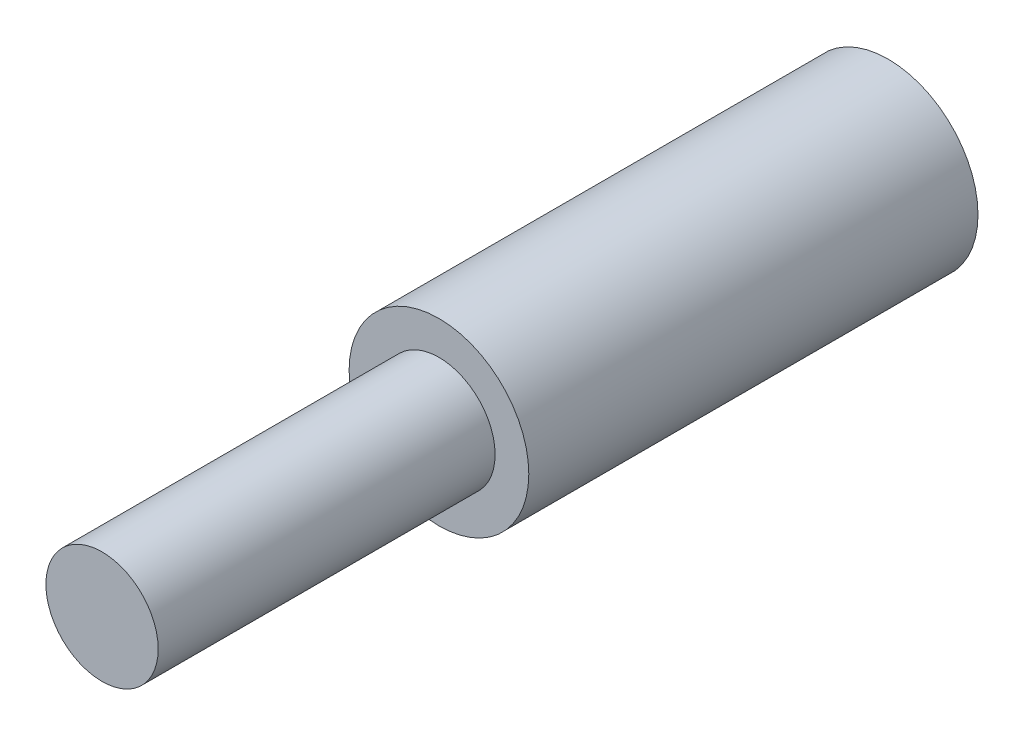
from build123d import *

# Parameters (mm, degrees)
SKETCH1_R           = 8
BOSS_EXTRUDE1_DEPTH = 40
SKETCH2_R           = 5
BOSS_EXTRUDE2_DEPTH = 30


with BuildPart() as part:
    # Sketch1 → Boss-Extrude1 (new body)
    with BuildSketch(Plane.XY):
        Circle(SKETCH1_R)
    extrude(amount=BOSS_EXTRUDE1_DEPTH)

    # Sketch2 → Boss-Extrude2 (add)
    with BuildSketch(Plane.XY.offset(40)):
        Circle(SKETCH2_R)
    extrude(amount=BOSS_EXTRUDE2_DEPTH)


solid = part.part
